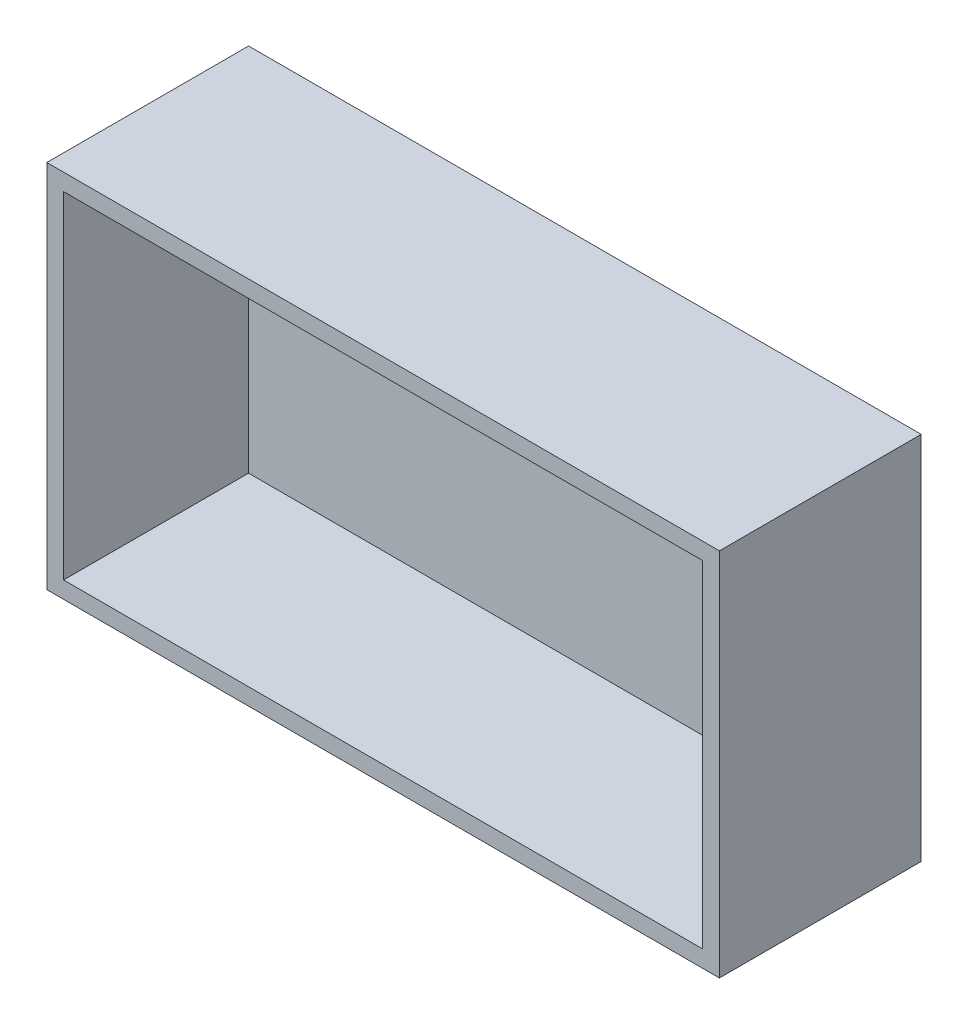
SolidWorks part; units mm, degrees
material "瓦楞纸板盒"
ref_plane "前视基准面" through (0, 0, 0) normal (0, 0, 1) x (1, 0, 0)
ref_plane "上视基准面" through (0, 0, 0) normal (0, 1, 0) x (1, 0, 0)
ref_plane "右视基准面" through (0, 0, 0) normal (1, 0, 0) x (0, 0, -1)
other "Configuration Table"
sketch "草图1" plane through (0, 0, 0) normal (0, 0, 1) x (1, 0, 0)
  line L1 (-190, -100) -> (190, -100)
  line L2 (-190, -100) -> (-190, 100)
  line L3 (-190, 100) -> (190, 100)
  line L4 (190, -100) -> (190, 100)
  line L5 (-190, -100) -> (190, 100) construction
  line L6 (-190, 100) -> (190, -100) construction
  point P0 (0, 0)
  dimension "D1" = 380
  dimension "D2" = 200
extrude "拉伸-薄壁1" add sketch "草图1" along normal blind 120 thin
sketch "草图2" plane through (0, 100, 0) normal (0, -1, 0) x (-1, 0, 0)
  line L0 (-200, -120) -> (-200, 0) construction
  line L1 (200, 0) -> (-200, 0)
  line L2 (200, 0) -> (200, -10)
  line L3 (200, -10) -> (-200, -10)
  line L4 (-200, 0) -> (-200, -10)
  dimension "D1" = 10
extrude "凸台-拉伸2" add sketch "草图2" along normal up to surface (210 mm away) up to face at (0, -110, 60)
